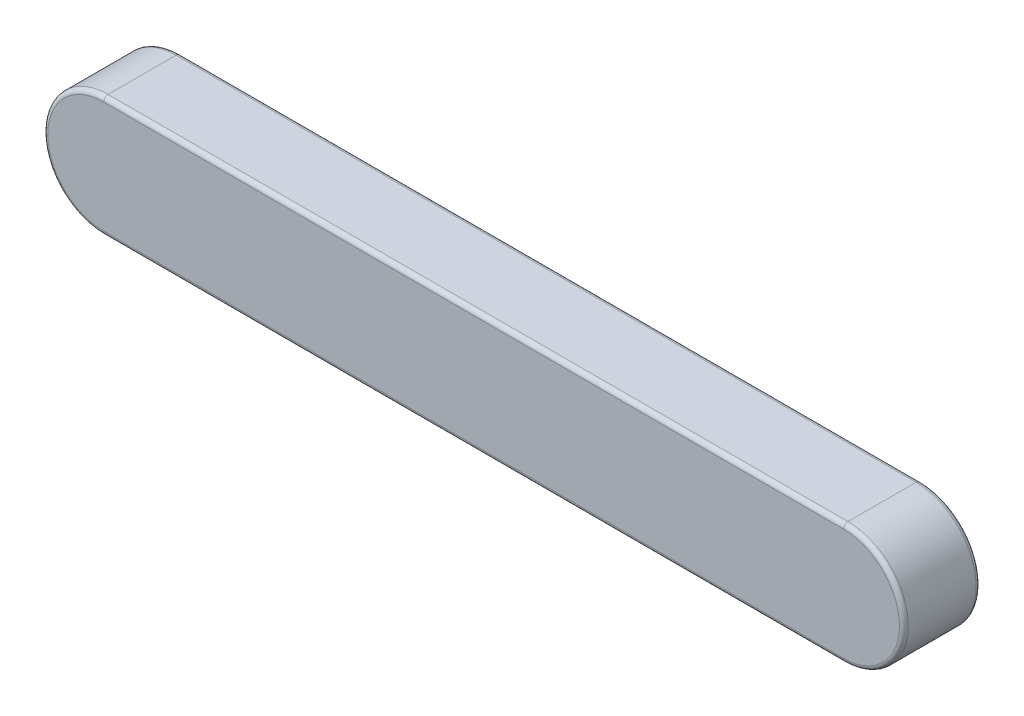
from build123d import *

# Parameters (mm, degrees)
BOSS_EXTRUDE1_DEPTH = 14
FILLET1_R           = 0.8


with BuildPart() as part:
    # Sketch1 → Boss-Extrude1 (new body)
    with BuildSketch(Plane.XY):
        with BuildLine():
            Line((-67.5, 11), (67.5, 11))
            ThreePointArc((67.5, 11), (78.5, 0), (67.5, -11))
            Line((67.5, -11), (-67.5, -11))
            ThreePointArc((-67.5, -11), (-78.5, 0), (-67.5, 11))
        make_face()
    extrude(amount=BOSS_EXTRUDE1_DEPTH)

    # Fillet1
    fillet1_edges = [part.edges().sort_by_distance(p)[0] for p in [
        (78.5, 0, 14),
        (0, 11, 14),
        (-78.5, 0, 14),
        (0, 11, 0),
        (78.5, 0, 0),
        (0, -11, 0),
        (-78.5, 0, 0),
        (0, -11, 14),
    ]]
    fillet(fillet1_edges, radius=FILLET1_R)


solid = part.part
